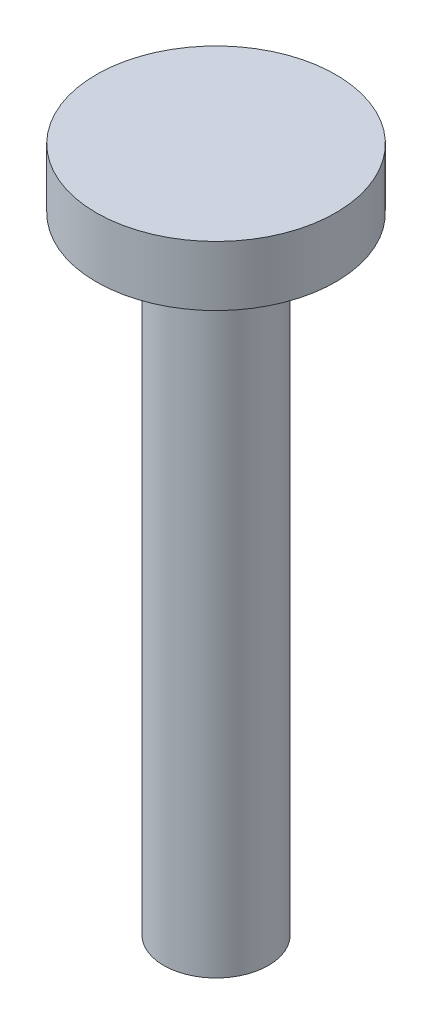
from build123d import *


with BuildPart() as part:
    # Sketch1 → Revolve1 (revolve)
    with BuildSketch(Plane.XY, mode=Mode.PRIVATE) as revolve1_sk:
        Polygon((0, 30), (4, 30), (4, 28), (1.75, 27.100495725), (1.75, 7.100495725), (0, 7.100495725), align=None)
    revolve(revolve1_sk.sketch.rotate(Axis((0, 30, 0), (0, -1, 0)), 90), axis=Axis((0, 30, 0), (0, -1, 0)))


solid = part.part
